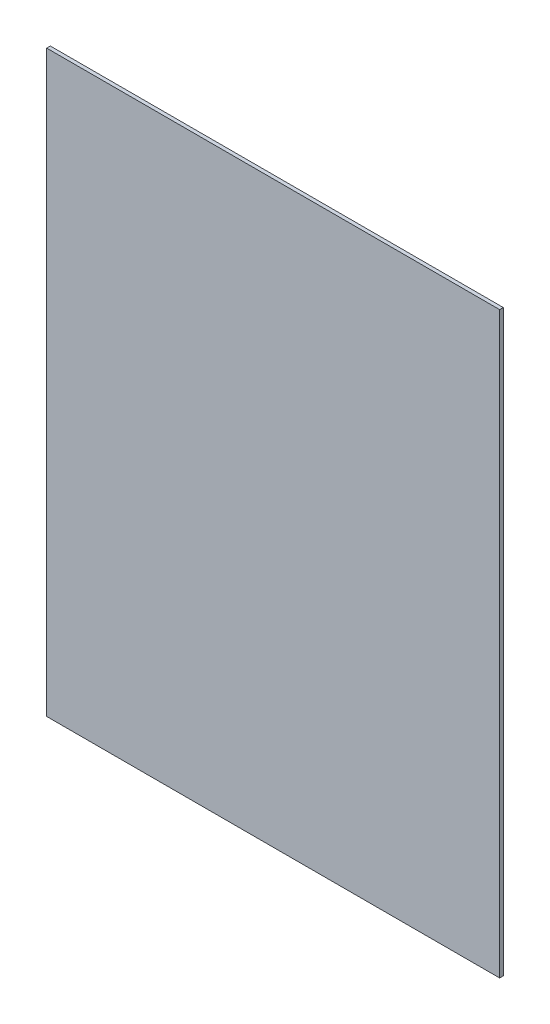
from build123d import *

# Parameters (mm, degrees)
SKETCH_1_W      = 619
SKETCH_1_H      = 791
EXTRUDE_1_DEPTH = 5


with BuildPart() as part:
    # 草图1 → 凸台-拉伸1 (new body)
    with BuildSketch(Plane.XY):
        Rectangle(SKETCH_1_W, SKETCH_1_H)
    extrude(amount=EXTRUDE_1_DEPTH)


solid = part.part
